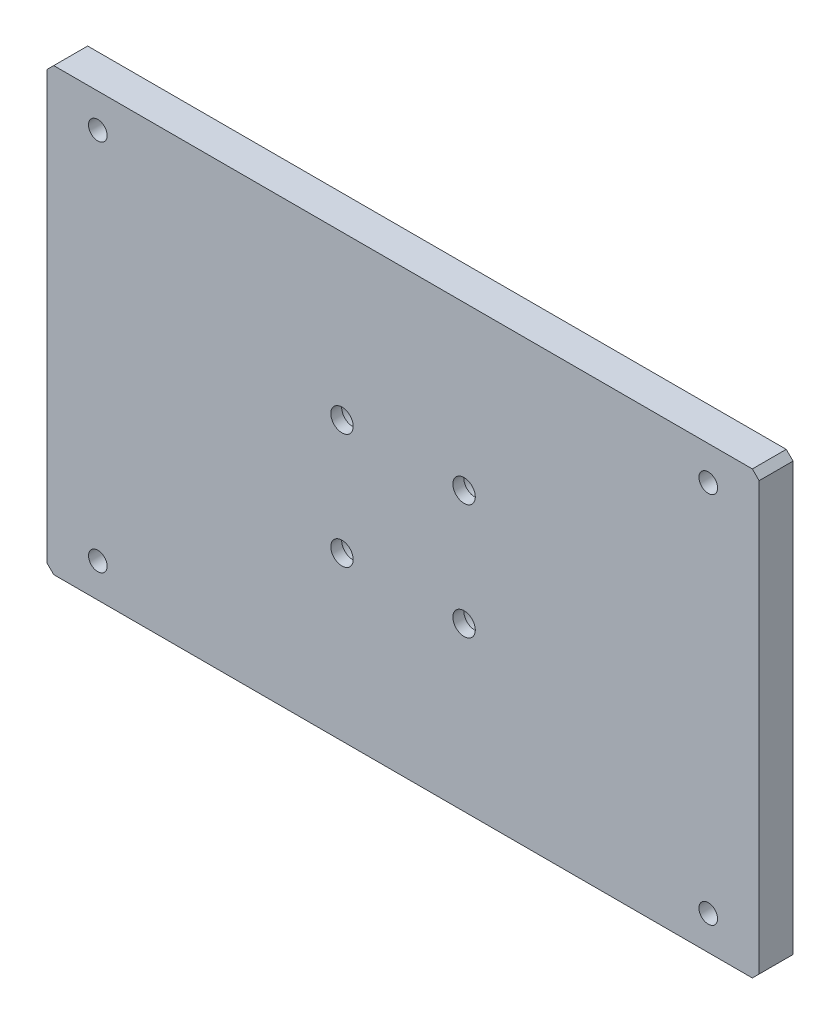
SolidWorks part; units mm, degrees
ref_plane "Front Plane" through (0, 0, 0) normal (0, 0, 1) x (1, 0, 0)
ref_plane "Top Plane" through (0, 0, 0) normal (0, 1, 0) x (1, 0, 0)
ref_plane "Right Plane" through (0, 0, 0) normal (1, 0, 0) x (0, 0, -1)
sketch "Sketch1" plane through (0, 0, 0) normal (0, 0, 1) x (1, 0, 0)
  line L1 (-105, -65) -> (105, -65)
  line L2 (-105, -65) -> (-105, 65)
  line L3 (-105, 65) -> (105, 65)
  line L4 (105, -65) -> (105, 65)
  line L5 (-105, -65) -> (105, 65) construction
  line L6 (-105, 65) -> (105, -65) construction
  point P0 (0, 0)
  dimension "D1" = 210
  dimension "D2" = 130
extrude "Boss-Extrude1" add sketch "Sketch1" along normal blind 10
sketch "Sketch2" [suppressed] plane through (0, 0, 10) normal (0, 0, 1) x (1, 0, 0)
  line L0 (-122.0076, 0) -> (116.5676, 0) construction
  line L1 (0, 81.5601) -> (0, -104.8714) construction
  line L2 (-85, 10) -> (-55, 10) construction
  line L3 (-85, 12) -> (-55, 12)
  line L4 (-85, 8) -> (-55, 8)
  line L5 (-30, 55) -> (-30, 25) construction
  line L8 (-28, 55) -> (-28, 25)
  line L9 (-32, 55) -> (-32, 25)
  line L11 (-85, -10) -> (-55, -10) construction
  line L12 (-85, -12) -> (-55, -12)
  line L13 (-85, -8) -> (-55, -8)
  line L14 (30, 55) -> (30, 25) construction
  line L15 (28, 55) -> (28, 25)
  line L16 (32, 55) -> (32, 25)
  line L17 (-30, -55) -> (-30, -25) construction
  line L18 (-28, -55) -> (-28, -25)
  line L19 (-32, -55) -> (-32, -25)
  line L20 (30, -55) -> (30, -25) construction
  line L21 (28, -55) -> (28, -25)
  line L22 (32, -55) -> (32, -25)
  line L23 (85, 10) -> (55, 10) construction
  line L24 (85, 12) -> (55, 12)
  line L25 (85, 8) -> (55, 8)
  line L26 (85, -10) -> (55, -10) construction
  line L27 (85, -12) -> (55, -12)
  line L28 (85, -8) -> (55, -8)
  arc A0 (-85, 12) -> (-85, 8) centre (-85, 10) ccw
  arc A1 (-55, 8) -> (-55, 12) centre (-55, 10) ccw
  arc A4 (-28, 55) -> (-32, 55) centre (-30, 55) ccw
  arc A5 (-32, 25) -> (-28, 25) centre (-30, 25) ccw
  arc A6 (-85, -12) -> (-85, -8) centre (-85, -10) cw
  arc A7 (-55, -8) -> (-55, -12) centre (-55, -10) cw
  arc A8 (28, 55) -> (32, 55) centre (30, 55) cw
  arc A9 (32, 25) -> (28, 25) centre (30, 25) cw
  arc A10 (-28, -55) -> (-32, -55) centre (-30, -55) cw
  arc A11 (-32, -25) -> (-28, -25) centre (-30, -25) cw
  arc A12 (28, -55) -> (32, -55) centre (30, -55) ccw
  arc A13 (32, -25) -> (28, -25) centre (30, -25) ccw
  arc A14 (85, 12) -> (85, 8) centre (85, 10) cw
  arc A15 (55, 8) -> (55, 12) centre (55, 10) cw
  arc A16 (85, -12) -> (85, -8) centre (85, -10) ccw
  arc A17 (55, -8) -> (55, -12) centre (55, -10) ccw
  point P7 (-70, 10)
  point P14 (-30, 40)
  point P21 (-70, -10)
  point P28 (30, 40)
  point P35 (-30, -40)
  point P42 (30, -40)
  point P49 (70, 10)
  point P56 (70, -10)
  dimension "D1" = 30
  dimension "D2" = 70
  dimension "D3" = 10
  dimension "D4" = 4
  dimension "D5" = 4
  dimension "D6" = 30
  dimension "D7" = 30
  dimension "D8" = 40
sketch "Sketch3" plane through (0, 0, 0) normal (0, 0, -1) x (-1, 0, 0)
  line L1 (18, -17) -> (-18, -17)
  line L2 (18, -17) -> (18, 17)
  line L3 (18, 17) -> (-18, 17)
  line L4 (-18, -17) -> (-18, 17)
  line L5 (90, -55) -> (-90, -55)
  line L6 (90, -55) -> (90, 55)
  line L7 (90, 55) -> (-90, 55)
  line L8 (-90, -55) -> (-90, 55)
hole_wizard "Hole size (per socket head cap screw type)1" positions "3DSketch1" profile "Sketch4" counterbore size "M6" standard "GB" end condition through all
sketch3d "3DSketch1"
  point P0 (-18, -17, 0)
  point P3 (18, -17, 0)
  point P6 (18, 17, 0)
  point P9 (-18, 17, 0)
sketch "Sketch4" plane through (-18, -17, 0) normal (1, 0, 0) x (0, 1, 0)
  line L0 (0, 0) -> (0, 10)
  line L1 (0, 10) -> (3.3, 10)
  line L3 (3.3, 10) -> (3.3, 6.8)
  line L4 (3.3, 6.8) -> (5.5, 6.8)
  line L5 (5.5, 6.8) -> (5.5, 0)
  line L7 (5.5, 0) -> (0, 0)
  line L11 (0, -6.35) -> (0, 107.95) construction
  dimension "通孔孔直径" = 6.6
  dimension "通孔孔深度" = 10
  dimension "柱形沉头孔直径" = 11
  dimension "柱形沉头孔深度" = 6.8
hole_wizard "Hole size (per socket head cap screw type)2" positions "3DSketch2" profile "Sketch5" counterbore size "M5" standard "GB" end condition through all
sketch3d "3DSketch2"
  point P0 (-90, -55, 0)
  point P3 (-90, 55, 0)
  point P6 (90, 55, 0)
  point P9 (90, -55, 0)
sketch "Sketch5" plane through (-90, -55, 0) normal (1, 0, 0) x (0, 1, 0)
  line L0 (0, 0) -> (0, 10)
  line L1 (0, 10) -> (2.75, 10)
  line L3 (2.75, 10) -> (2.75, 5.7)
  line L4 (2.75, 5.7) -> (5, 5.7)
  line L5 (5, 5.7) -> (5, 0)
  line L7 (5, 0) -> (0, 0)
  line L11 (0, -6.35) -> (0, 107.95) construction
  dimension "通孔孔直径" = 5.5
  dimension "通孔孔深度" = 10
  dimension "柱形沉头孔直径" = 10
  dimension "柱形沉头孔深度" = 5.7
chamfer "Chamfer1" distance 2 angle 45 4 edges at (-105, -65, 5) (-105, 65, 5) (105, -65, 5) (105, 65, 5)
